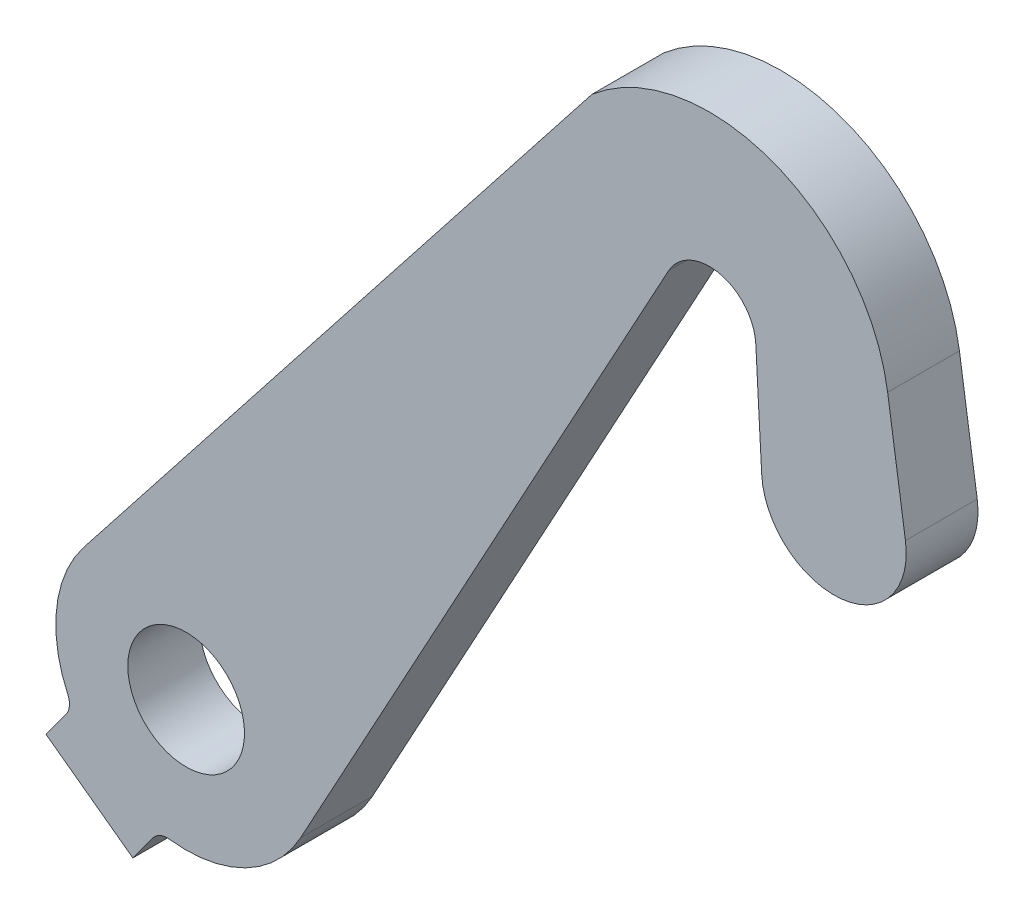
from build123d import *

# Parameters (mm, degrees)
SKETCH1_R           = 6.5
BOSS_EXTRUDE1_DEPTH = 4
FILLET1_R           = 2


with BuildPart() as part:
    # Sketch1 → Boss-Extrude1 (new, symmetric)
    with BuildSketch(Plane.XY):
        with BuildLine():
            Line((47.613190214, 66.596790509), (6.61525122, -8.614210923))
            ThreePointArc((6.61525122, -8.614210923), (-0.051073307, -14.850717485), (-9.121738509, -15.878788295))
            Line((-9.121738509, -15.878788295), (-12.077727744, -19.911421137))
            Line((-12.077727744, -19.911421137), (-21.756046565, -12.817046972))
            Line((-21.756046565, -12.817046972), (-18.80005733, -8.784414129))
            ThreePointArc((-18.80005733, -8.784414129), (-20.623291354, -0.545508517), (-17.559429464, 7.316838354))
            Line((-17.559429464, 7.316838354), (39.076322986, 79.353992026))
            ThreePointArc((39.076322986, 79.353992026), (59.174366459, 82.937056923), (72.02582234, 67.074844364))
            Line((72.02582234, 67.074844364), (74.007984491, 53.75944084))
            ThreePointArc((74.007984491, 53.75944084), (66.847485005, 44.555404253), (57.99070376, 52.141211286))
            Line((57.99070376, 52.141211286), (57.333258746, 64.39522394))
            ThreePointArc((57.333258746, 64.39522394), (53.305241341, 69.169419157), (47.613190214, 66.596790509))
        make_face()
        with Locations((-6.139534384, -1.661505705)):
            Circle(SKETCH1_R, mode=Mode.SUBTRACT)
    extrude(amount=BOSS_EXTRUDE1_DEPTH, both=True)

    # Fillet1
    fillet1_edges = [part.edges().sort_by_distance(p)[0] for p in [
        (-18.80005733, -8.784414129, 0),
        (-9.121738509, -15.878788295, 0),
    ]]
    fillet(fillet1_edges, radius=FILLET1_R)


solid = part.part
